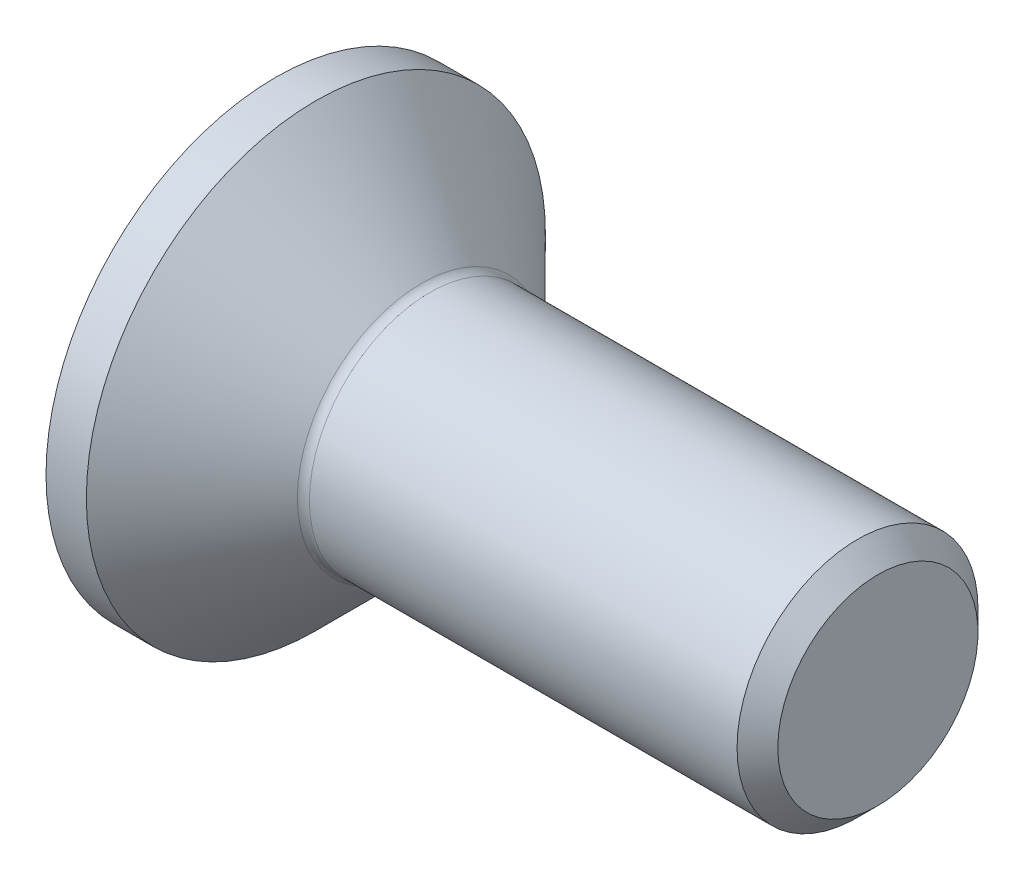
SolidWorks part; units mm, degrees
ref_plane "Front" through (0, 0, 0) normal (0, 0, 1) x (1, 0, 0)
ref_plane "Top" through (0, 0, 0) normal (0, 1, 0) x (1, 0, 0)
ref_plane "Right" through (0, 0, 0) normal (1, 0, 0) x (0, 0, -1)
sketch "Sketch1" plane through (0, 0, 0) normal (0, 0, 1) x (1, 0, 0)
  line L0 (0, 0) -> (0, 8.96)
  line L1 (0, 8.96) -> (4.96, 4)
  line L2 (4.96, 4) -> (20, 4)
  line L3 (20, 4) -> (20, 0)
  line L4 (20, 0) -> (0, 0)
  line L5 (-0.5871, 0) -> (5.4927, 0) construction
  dimension "D1" = 45
  dimension "l" = 20
  dimension "k" = 4.96
  dimension "d" = 8
revolve "Base" add sketch "Sketch1" angle 360 about L5
cosmetic thread "ThreadCosmetic1" parameters "b"=15, "D2"=6.647
sketch "Sketch2" plane through (0, 0, 0) normal (1, 0, 0) x (0, 0, -1)
  line L1 (2.8868, 0) -> (1.4434, 2.5)
  line L2 (1.4434, 2.5) -> (-1.4434, 2.5)
  line L3 (-1.4434, 2.5) -> (-2.8868, 0)
  line L4 (-2.8868, 0) -> (-1.4434, -2.5)
  line L5 (-1.4434, -2.5) -> (1.4434, -2.5)
  line L6 (1.4434, -2.5) -> (2.8868, 0)
  circle A0 centre (0, 0) radius 2.5 construction
  dimension "s" = 5
extrude "HexagonSocket" cut sketch "Sketch2" along normal blind 3
sketch "Sketch3" plane through (0, 0, 0) normal (0, 0, 1) x (1, 0, 0)
  line L0 (-0.4391, 0) -> (4.425, 0) construction
  line L1 (3, 0) -> (3, -2.5) construction
  line L2 (3, 2.5) -> (4.4434, 0)
  line L3 (4.4434, 0) -> (3, -2.5) construction
  line L4 (3, 2.5) -> (3, 0)
  line L5 (3, 0) -> (4.4434, 0)
  line L7 (3, 2.5) -> (3, 0) construction
  dimension "D1" = 120
revolve "Cut-Revolve1" cut sketch "Sketch3" angle 360 about L0
fillet "HeadFillet" radius 0.4 1 edges at (4.96, 0, 4)
chamfer "Chamfer" distance 0.6765 angle 45 1 edges at (20, 0, 4)
sketch "Sketch4" plane through (0, 0, 0) normal (0, 1, 0) x (1, 0, 0)
  line L0 (11.8531, 0) -> (-2.694, 0) construction
  line L1 (-2, 12.62) -> (3, 12.62)
  line L2 (-2, 12.62) -> (-2, 7.62)
  line L3 (-2, 7.62) -> (3, 7.62)
  line L4 (3, 12.62) -> (3, 7.62)
  line L5 (0, 8.96) -> (0, -8.96) construction
  dimension "dk" = 15.24
  dimension "D2" = 2
  dimension "D3" = 5
  dimension "D4" = 5
revolve "Cut-Revolve2" cut sketch "Sketch4" angle 360 about L0
sketch "Sketch5" plane through (0, 0, 0) normal (0, 0, 1) x (1, 0, 0)
  line L0 (19.3235, 3.4141) -> (19.6617, 4)
  line L1 (19.6617, 4) -> (19.6617, 4.6765)
  line L2 (19.6617, 4.6765) -> (18.9853, 4.6765)
  line L3 (18.9853, 4.6765) -> (18.9853, 4)
  line L4 (18.9853, 4) -> (19.3235, 3.4141)
  line L5 (0, 0) -> (10.6885, 0) construction
  line L6 (19.3235, 4) -> (19.3235, -4) construction
  dimension "D1" = 8
  dimension "D2" = 0.6765
revolve "Cut-Revolve10" [suppressed] cut sketch "Sketch5" angle 360 about L5
pattern_linear "LPattern10" [suppressed] count 18 spacing 0.8118 along (1, 0, 0)
equation "\"D1@Chamfer\" = (  \"d@Sketch1\" - \"D2@ThreadCosmetic1\" )  / 2"
equation "\"D1@Sketch5\" = \"d@Sketch1\""
equation "\"D2@Sketch5\" =  ( \"d@Sketch1\" - \"D2@ThreadCosmetic1\" )  / 2"
equation "\"D3@LPattern10\" = \"D2@Sketch5\" * 1.2"
equation "\"D1@LPattern10\" = \"b@ThreadCosmetic1\" / \"D3@LPattern10\""
